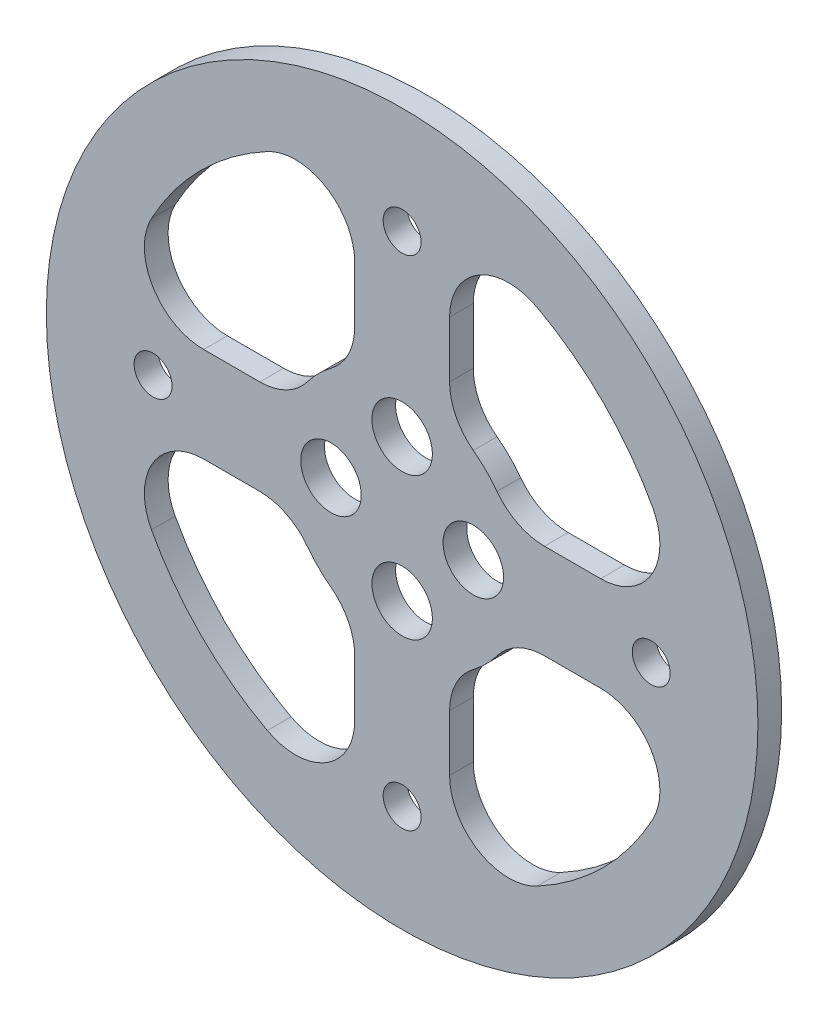
SolidWorks part; units mm, degrees
material "Thornel Mat VMA"
ref_plane "前视基准面" through (0, 0, 0) normal (0, 0, 1) x (1, 0, 0)
ref_plane "上视基准面" through (0, 0, 0) normal (0, 1, 0) x (1, 0, 0)
ref_plane "右视基准面" through (0, 0, 0) normal (1, 0, 0) x (0, 0, -1)
sketch "草图1" plane through (0, 0, 0) normal (0, 0, 1) x (1, 0, 0)
  line L0 (0, 0) -> (24, 0) construction
  line L14 (4, 16.7332) -> (4, 12)
  line L15 (-4, 16.7332) -> (-4, 12)
  line L16 (16.7332, 4) -> (12, 4)
  line L17 (16.7332, -4) -> (12, -4)
  line L18 (4, -16.7332) -> (4, -12)
  line L19 (-4, -16.7332) -> (-4, -12)
  line L20 (-16.7332, -4) -> (-12, -4)
  line L21 (-16.7332, 4) -> (-12, 4)
  circle A0 centre (0, 0) radius 30
  arc A1 (-11.3684, 21.1367) -> (-21.1367, 11.3684) centre (0, 0) ccw
  arc A19 (-6, 8) -> (-8, 6) centre (0, 0) ccw
  arc A33 (4, 12) -> (6, 8) centre (9, 12) ccw
  arc A34 (-4, 12) -> (-6, 8) centre (-9, 12) cw
  arc A35 (4, 16.7332) -> (11.3684, 21.1367) centre (9, 16.7332) cw
  arc A36 (-4, 16.7332) -> (-11.3684, 21.1367) centre (-9, 16.7332) ccw
  arc A37 (16.7332, 4) -> (21.1367, 11.3684) centre (16.7332, 9) ccw
  arc A38 (12, 4) -> (8, 6) centre (12, 9) cw
  arc A39 (16.7332, -4) -> (21.1367, -11.3684) centre (16.7332, -9) cw
  arc A40 (12, -4) -> (8, -6) centre (12, -9) ccw
  arc A41 (4, -16.7332) -> (11.3684, -21.1367) centre (9, -16.7332) ccw
  arc A42 (4, -12) -> (6, -8) centre (9, -12) cw
  arc A43 (-4, -16.7332) -> (-11.3684, -21.1367) centre (-9, -16.7332) cw
  arc A44 (-4, -12) -> (-6, -8) centre (-9, -12) ccw
  arc A45 (-16.7332, -4) -> (-21.1367, -11.3684) centre (-16.7332, -9) ccw
  arc A46 (-12, -4) -> (-8, -6) centre (-12, -9) cw
  arc A47 (-16.7332, 4) -> (-21.1367, 11.3684) centre (-16.7332, 9) cw
  arc A48 (-12, 4) -> (-8, 6) centre (-12, 9) ccw
  arc A49 (-8, -6) -> (-6, -8) centre (0, 0) ccw
  arc A50 (-21.1367, -11.3684) -> (-11.3684, -21.1367) centre (0, 0) ccw
  arc A51 (6, -8) -> (8, -6) centre (0, 0) ccw
  arc A52 (8, 6) -> (6, 8) centre (0, 0) ccw
  arc A53 (11.3684, -21.1367) -> (21.1367, -11.3684) centre (0, 0) ccw
  arc A54 (21.1367, 11.3684) -> (11.3684, 21.1367) centre (0, 0) ccw
  point P15 (0, 0)
  point P40 (0, 0)
  point P51 (0, 0)
  point P94 (0, 0)
  dimension "D1" = 60
  dimension "D2" = 24
  dimension "D5" = 8
  dimension "D6" = 5
  dimension "D8" = 10
  dimension "D7" = 4
extrude "凸台-拉伸1" add sketch "草图1" along normal blind 2
sketch "草图2" plane through (0, 0, 2) normal (0, 0, 1) x (1, 0, 0)
  circle A0 centre (0, 0) radius 21 construction
  circle A1 centre (-21, 0) radius 1.6
  circle A2 centre (0, 21) radius 1.6
  circle A3 centre (21, 0) radius 1.6
  circle A4 centre (0, -21) radius 1.6
  point P14 (0, 0)
  dimension "D1" = 42
  dimension "D2" = 3.2
  dimension "D3" = 4
extrude "切除-拉伸1" cut sketch "草图2" against normal blind 10
sketch "草图3" plane through (0, 0, 2) normal (0, 0, 1) x (1, 0, 0)
  line L0 (0, 6) -> (-6, 0) construction
  line L1 (0, 6) -> (6, 0) construction
  line L2 (-6, 0) -> (0, -6) construction
  line L3 (6, 0) -> (0, -6) construction
  line L4 (-6, 0) -> (6, 0) construction
  line L5 (0, 6) -> (0, -6) construction
  circle A0 centre (0, 6) radius 2.55
  circle A1 centre (-6, 0) radius 2.55
  circle A2 centre (6, 0) radius 2.55
  circle A3 centre (0, -6) radius 2.55
  point P0 (0, 0)
  dimension "D2" = 5.1
  dimension "D1" = 6
extrude "切除-拉伸2" cut sketch "草图3" against normal blind 10
